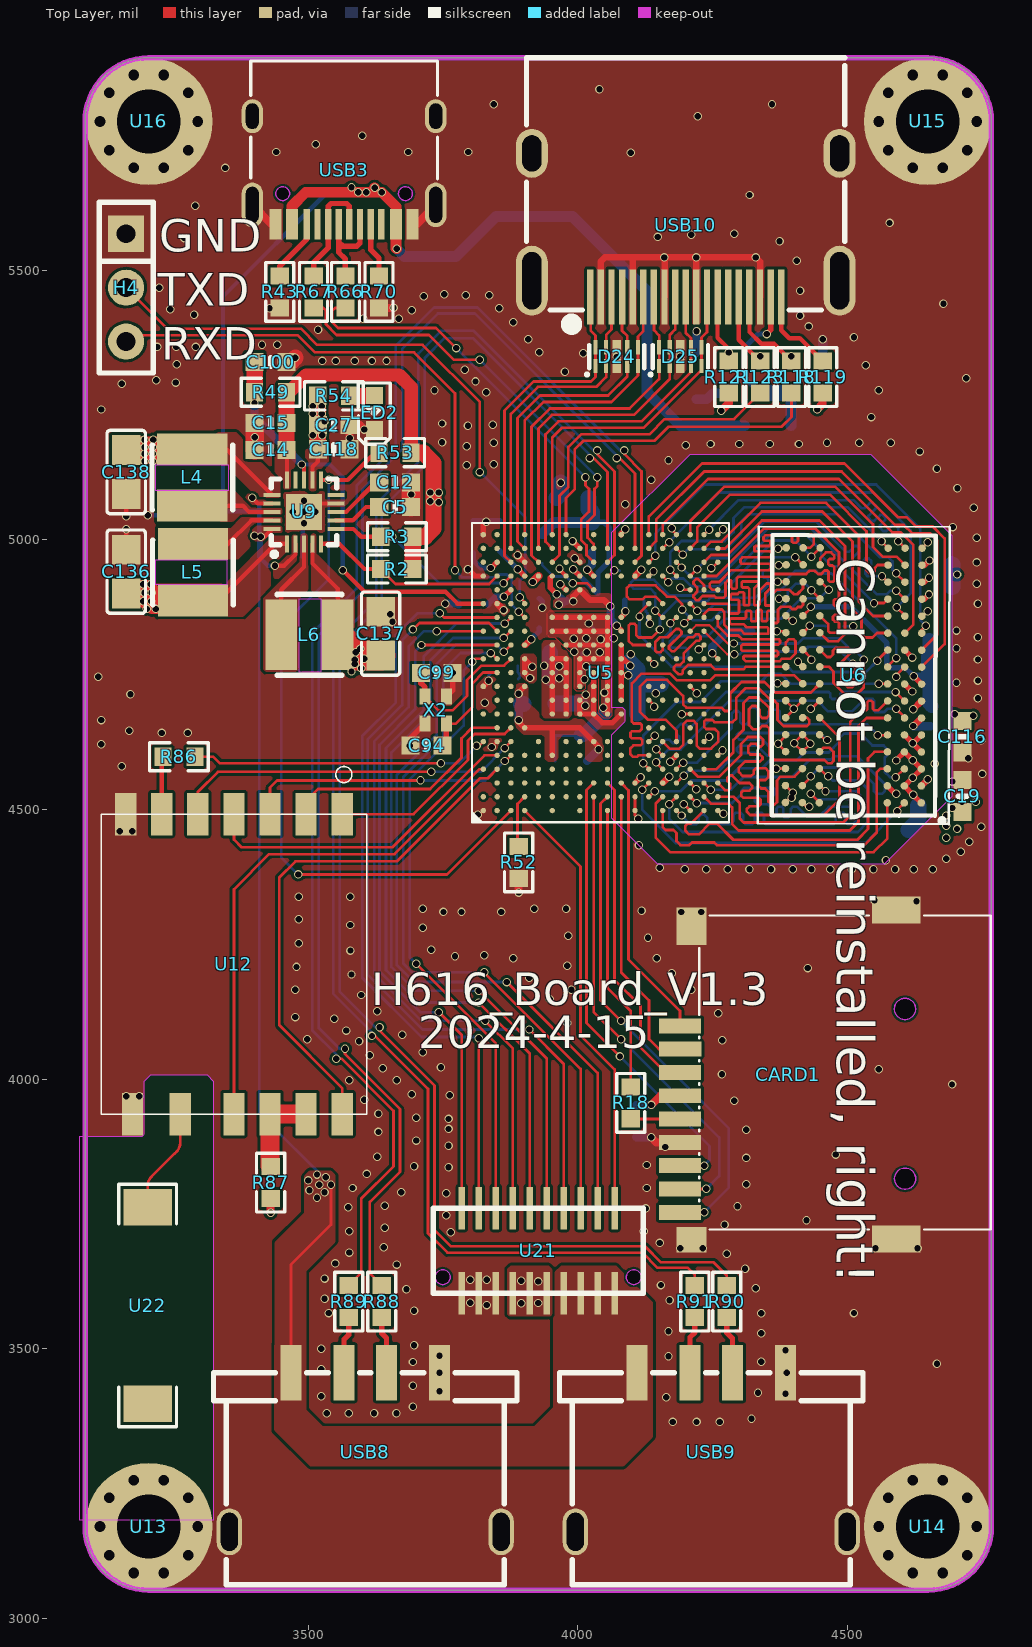
[diagram p0: Top Layer view]
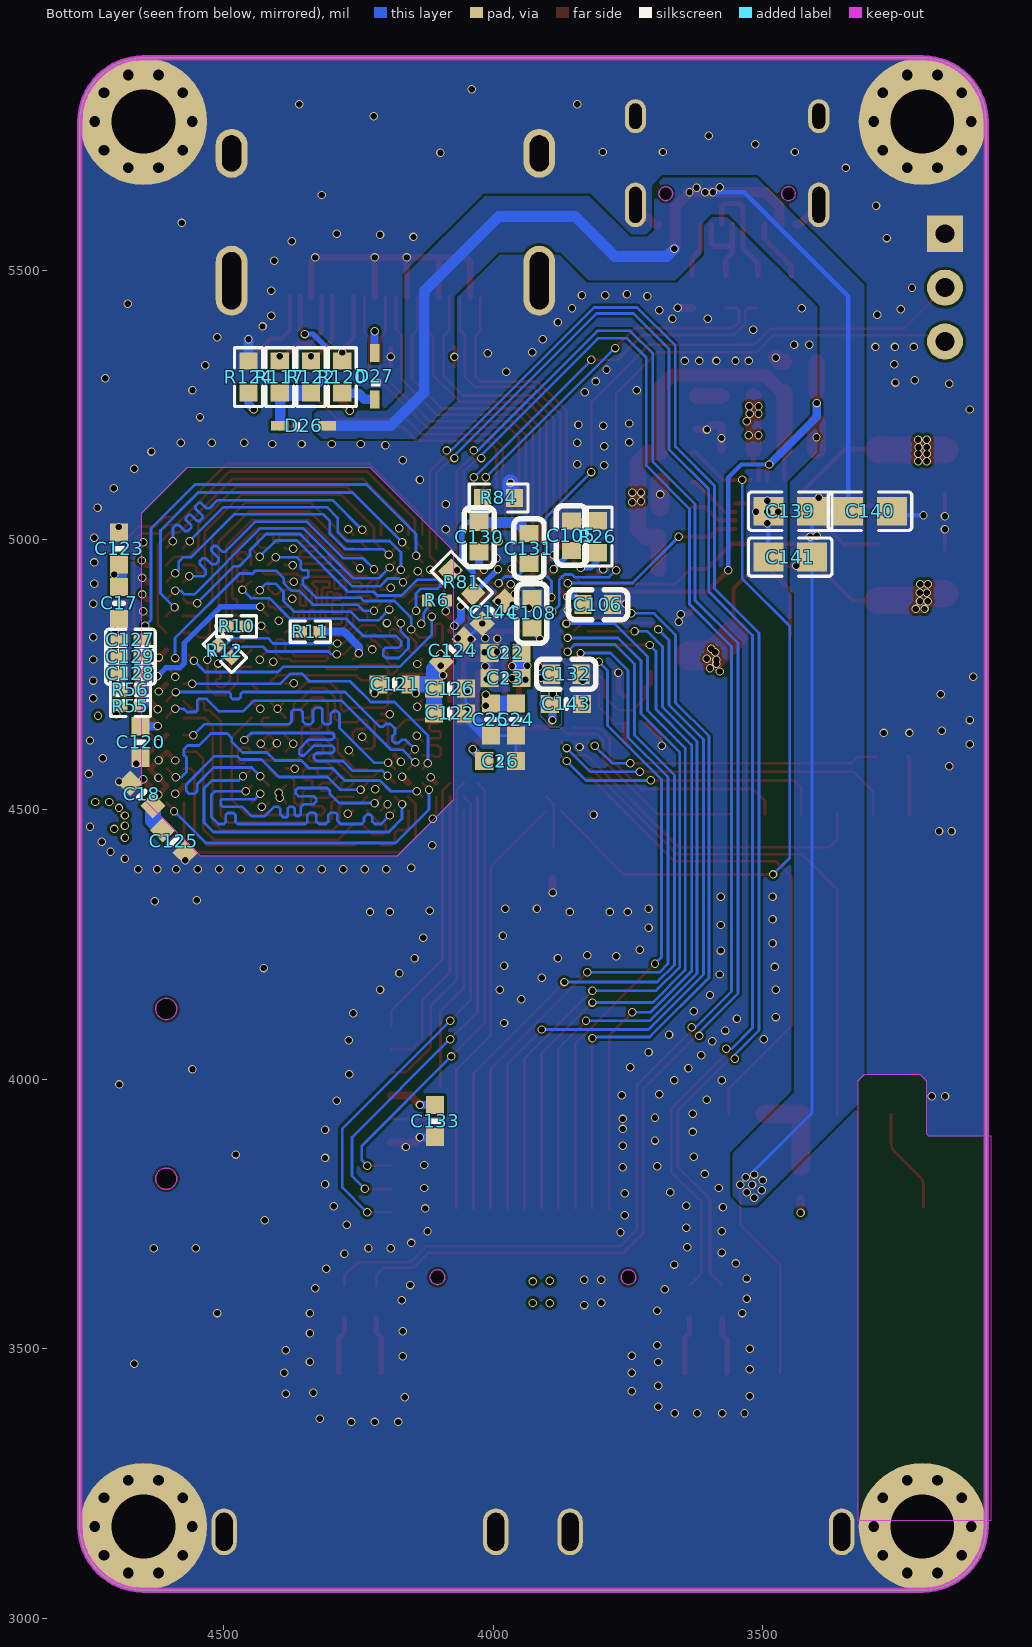
[diagram p1: Bottom Layer view, seen from below]
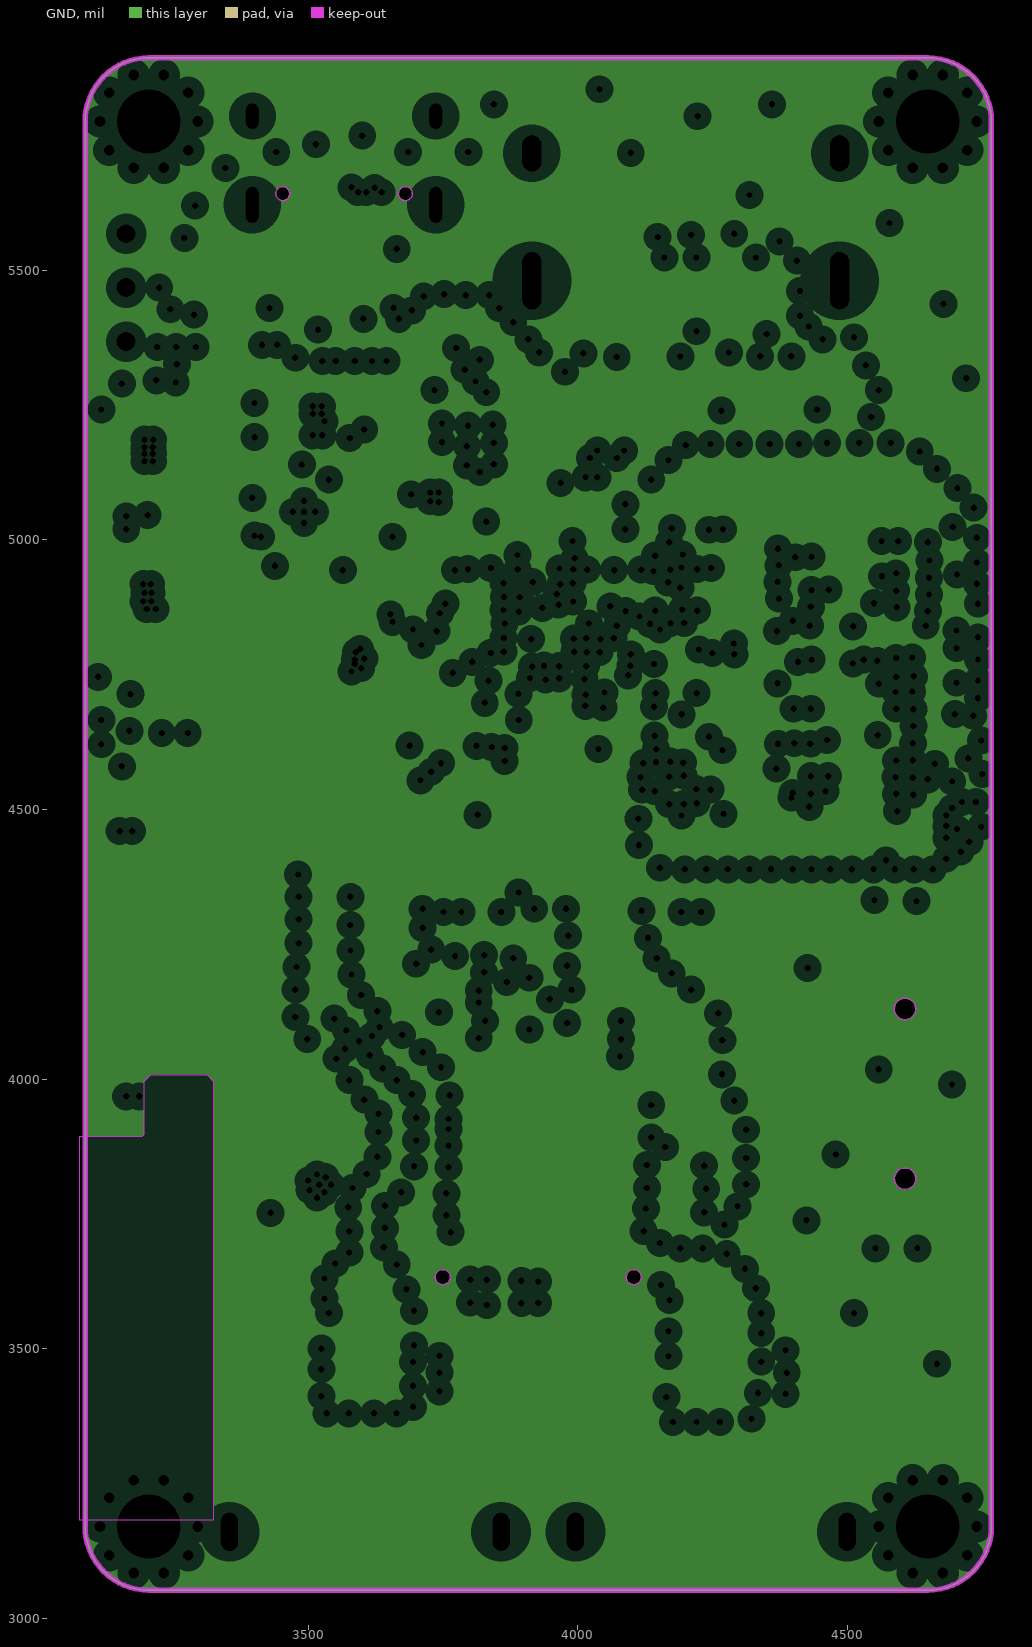
[diagram p2: GND, clearances drawn from the general rule]
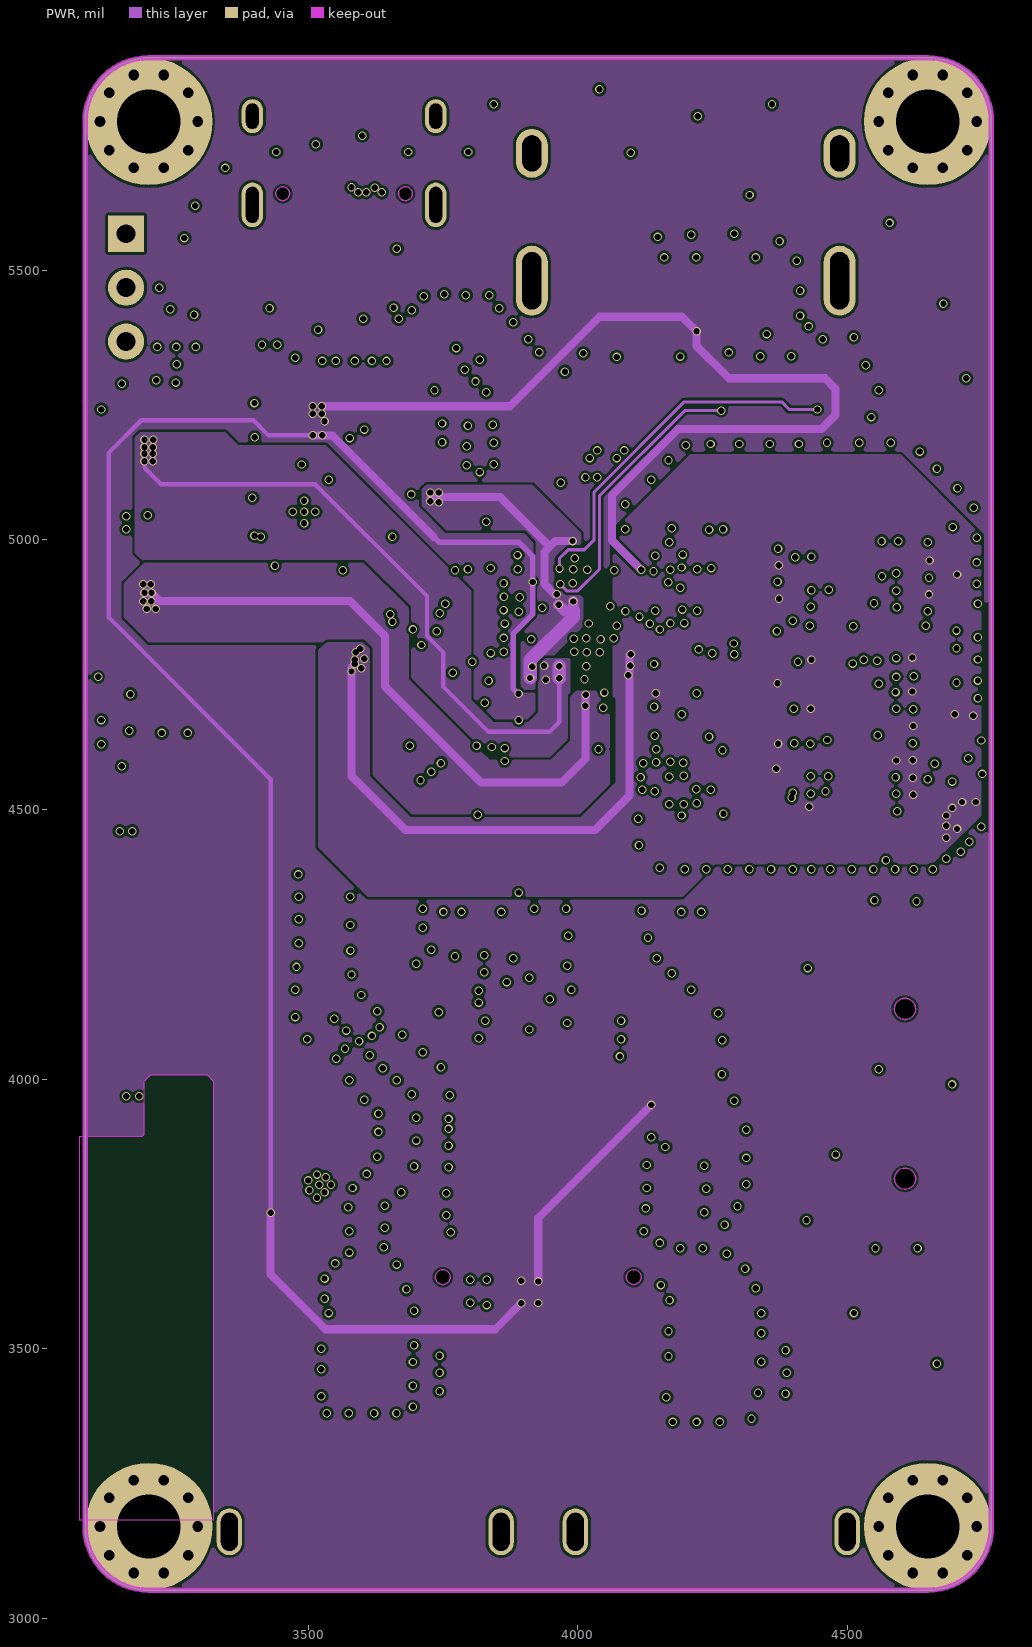
[diagram p3: PWR]
# Altium PCB MISC105417.pcbdoc (part 1 of 5)
Units mil, origin at the board's own origin, x right, y up, seen from the top; angles counter-clockwise.
Board outline 1681.1 x 2842.52 mil, 4 copper layers (Top Layer, GND, PWR, Bottom Layer), stack 62.447 mil thick; 102 components, 152 nets, 737 pads, 611 vias.

## Layer stack, top to bottom
Top Layer: signal copper 1.378
Dielectric1: surface 8.283, 7628 RC49% 8.6mil, Dk 0
GND: plane copper 0.598
Dielectric2: surface 41.929, 1.1mm H/HOZ 含铜, Dk 0
PWR: signal copper 0.598
Dielectric3: surface 8.283, 7628 RC49% 8.6mil, Dk 0
Bottom Layer: signal copper 1.378

## Board outline
3204,5894.41 ccw(c3204,5776.3) 3085.89,5776.3 3085.89,3170 ccw(c3204,3170) 3204,3051.89 4648.88,3051.89 ccw(c4648.88,3170) 4766.99,3170 4766.99,5776.3 ccw(c4648.88,5776.3) 4648.88,5894.41 3204,5894.41

## Design rules (kind name [scope] priority, off if disabled: settings)
BoardOutlineClearance safeClearance_1 [All] p2 off: genericclearance=3.5 ignorepadtopadclearanceinfootprint=FALSE except(0: Arc-SplitContinuation Track-SplitContinuation SMDPad-SplitContinuation THPad-SplitContinuation Via-SplitContinuation Fill-SplitContinuation Region-SplitContinuation Poly-SplitContinuation Text-SplitContinuation Hole-SplitContinuation; 4: Arc-OutlineEdge Track-OutlineEdge SMDPad-OutlineEdge THPad-OutlineEdge Via-OutlineEdge Fill-OutlineEdge Region-OutlineEdge Text-OutlineEdge Hole-OutlineEdge Arc-CutoutEdge Track-CutoutEdge SMDPad-CutoutEdge THPad-CutoutEdge Via-CutoutEdge Fill-CutoutEdge Region-CutoutEdge Text-CutoutEdge Hole-CutoutEdge; 5: Poly-OutlineEdge Poly-CutoutEdge)
BoardOutlineClearance copperThicknessInner0.5oz_1 [All] p4 off: genericclearance=3.5 ignorepadtopadclearanceinfootprint=FALSE except(0: Arc-SplitContinuation Track-SplitContinuation SMDPad-SplitContinuation THPad-SplitContinuation Via-SplitContinuation Fill-SplitContinuation Region-SplitContinuation Poly-SplitContinuation Text-SplitContinuation Hole-SplitContinuation; 4: Arc-OutlineEdge Track-OutlineEdge SMDPad-OutlineEdge THPad-OutlineEdge Via-OutlineEdge Fill-OutlineEdge Region-OutlineEdge Text-OutlineEdge Hole-OutlineEdge Arc-CutoutEdge Track-CutoutEdge SMDPad-CutoutEdge THPad-CutoutEdge Via-CutoutEdge Fill-CutoutEdge Region-CutoutEdge Text-CutoutEdge Hole-CutoutEdge; 5: Poly-OutlineEdge Poly-CutoutEdge)
BoardOutlineClearance Plane_innerPlane_1 [All] p6 off: genericclearance=4 ignorepadtopadclearanceinfootprint=FALSE except(0: Arc-SplitContinuation Track-SplitContinuation SMDPad-SplitContinuation THPad-SplitContinuation Via-SplitContinuation Fill-SplitContinuation Region-SplitContinuation Poly-SplitContinuation Text-SplitContinuation Hole-SplitContinuation; 4: Arc-OutlineEdge Track-OutlineEdge SMDPad-OutlineEdge THPad-OutlineEdge Via-OutlineEdge Fill-OutlineEdge Region-OutlineEdge Text-OutlineEdge Hole-OutlineEdge Arc-CutoutEdge Track-CutoutEdge SMDPad-CutoutEdge THPad-CutoutEdge Via-CutoutEdge Fill-CutoutEdge Region-CutoutEdge Text-CutoutEdge Hole-CutoutEdge; 5: Poly-OutlineEdge Poly-CutoutEdge)
BoardOutlineClearance Copper_copperRegion_1 [All] p8 off: genericclearance=4 ignorepadtopadclearanceinfootprint=FALSE except(0: Arc-SplitContinuation Track-SplitContinuation SMDPad-SplitContinuation THPad-SplitContinuation Via-SplitContinuation Fill-SplitContinuation Region-SplitContinuation Poly-SplitContinuation Text-SplitContinuation Hole-SplitContinuation; 4: Arc-OutlineEdge Track-OutlineEdge SMDPad-OutlineEdge THPad-OutlineEdge Via-OutlineEdge Fill-OutlineEdge Region-OutlineEdge Text-OutlineEdge Hole-OutlineEdge Arc-CutoutEdge Track-CutoutEdge SMDPad-CutoutEdge THPad-CutoutEdge Via-CutoutEdge Fill-CutoutEdge Region-CutoutEdge Text-CutoutEdge Hole-CutoutEdge; 10: Poly-OutlineEdge Poly-CutoutEdge)
BoardOutlineClearance Copper_近距离铺铜_1 [All] p10 off: genericclearance=4 ignorepadtopadclearanceinfootprint=FALSE except(0: Arc-SplitContinuation Track-SplitContinuation SMDPad-SplitContinuation THPad-SplitContinuation Via-SplitContinuation Fill-SplitContinuation Region-SplitContinuation Poly-SplitContinuation Text-SplitContinuation Hole-SplitContinuation; 4: Arc-OutlineEdge Track-OutlineEdge SMDPad-OutlineEdge THPad-OutlineEdge Via-OutlineEdge Fill-OutlineEdge Region-OutlineEdge Text-OutlineEdge Hole-OutlineEdge Arc-CutoutEdge Track-CutoutEdge SMDPad-CutoutEdge THPad-CutoutEdge Via-CutoutEdge Fill-CutoutEdge Region-CutoutEdge Text-CutoutEdge Hole-CutoutEdge; 5: Poly-OutlineEdge Poly-CutoutEdge)
BoardOutlineClearance Copper_发散铺铜_1 [All] p12 off: genericclearance=4 ignorepadtopadclearanceinfootprint=FALSE except(0: Arc-SplitContinuation Track-SplitContinuation SMDPad-SplitContinuation THPad-SplitContinuation Via-SplitContinuation Fill-SplitContinuation Region-SplitContinuation Poly-SplitContinuation Text-SplitContinuation Hole-SplitContinuation; 4: Arc-OutlineEdge Track-OutlineEdge SMDPad-OutlineEdge THPad-OutlineEdge Via-OutlineEdge Fill-OutlineEdge Region-OutlineEdge Text-OutlineEdge Hole-OutlineEdge Arc-CutoutEdge Track-CutoutEdge SMDPad-CutoutEdge THPad-CutoutEdge Via-CutoutEdge Fill-CutoutEdge Region-CutoutEdge Text-CutoutEdge Hole-CutoutEdge; 5: Poly-OutlineEdge Poly-CutoutEdge)
BoardOutlineClearance copperThickness1oz_1 [All] p14: genericclearance=4 ignorepadtopadclearanceinfootprint=FALSE except(0: Arc-SplitContinuation Track-SplitContinuation SMDPad-SplitContinuation THPad-SplitContinuation Via-SplitContinuation Fill-SplitContinuation Region-SplitContinuation Poly-SplitContinuation Text-SplitContinuation Hole-SplitContinuation; 4: Arc-OutlineEdge Track-OutlineEdge SMDPad-OutlineEdge THPad-OutlineEdge Via-OutlineEdge Fill-OutlineEdge Region-OutlineEdge Text-OutlineEdge Hole-OutlineEdge Arc-CutoutEdge Track-CutoutEdge SMDPad-CutoutEdge THPad-CutoutEdge Via-CutoutEdge Fill-CutoutEdge Region-CutoutEdge Text-CutoutEdge Hole-CutoutEdge; 5: Poly-OutlineEdge Poly-CutoutEdge)
Clearance safeClearance [All] p1 off: gap=3.5 ignorepadtopadclearanceinfootprint=FALSE except(4: Track-Via SMDPad-Via THPad-Via Via-Via Fill-Track Region-Track Fill-SMDPad Region-SMDPad Fill-THPad Region-THPad Fill-Via Region-Via Fill-Fill Fill-Region Region-Region Arc-Track Arc-SMDPad Arc-THPad Arc-Via Fill-Arc Region-Arc Arc-Arc Text-Track SMDPad-Text Text-THPad Text-Via Fill-Text Region-Text Arc-Text Text-Text Hole-Via Fill-Hole Region-Hole Hole-Arc Hole-Text; 5: Poly-Track Poly-SMDPad Poly-THPad Poly-Via Poly-Fill Poly-Region Poly-Poly Poly-Arc Poly-Text Poly-Hole)
Clearance copperThicknessInner0.5oz [All] p3 off: gap=3.5 ignorepadtopadclearanceinfootprint=FALSE except(4: SMDPad-Track SMDPad-SMDPad THPad-Track SMDPad-THPad THPad-THPad Track-Via SMDPad-Via THPad-Via Via-Via Fill-Track Region-Track Fill-SMDPad Region-SMDPad Fill-THPad Region-THPad Fill-Via Region-Via Fill-Fill Fill-Region Region-Region Arc-Track Arc-SMDPad Arc-THPad Arc-Via Fill-Arc Region-Arc Arc-Arc Text-Track SMDPad-Text Text-THPad Text-Via Fill-Text Region-Text Arc-Text Text-Text Hole-Track Hole-SMDPad Hole-THPad Hole-Via Fill-Hole Region-Hole Hole-Arc Hole-Text; 5: Poly-Track Poly-SMDPad Poly-THPad Poly-Via Poly-Fill Poly-Region Poly-Poly Poly-Arc Poly-Text Poly-Hole)
Clearance Plane_innerPlane [All] p5 off: gap=4 ignorepadtopadclearanceinfootprint=FALSE except(5: Poly-Track Poly-SMDPad Poly-THPad Poly-Via Poly-Fill Poly-Region Poly-Poly Poly-Arc Poly-Text Poly-Hole)
Clearance Copper_copperRegion [All] p7 off: gap=4 ignorepadtopadclearanceinfootprint=FALSE except(10: Poly-Track Poly-SMDPad Poly-THPad Poly-Via Poly-Fill Poly-Region Poly-Poly Poly-Arc Poly-Text Poly-Hole)
Clearance Copper_近距离铺铜 [All] p9 off: gap=4 ignorepadtopadclearanceinfootprint=FALSE except(5: Poly-Track Poly-SMDPad Poly-THPad Poly-Via Poly-Fill Poly-Region Poly-Poly Poly-Arc Poly-Text Poly-Hole)
Clearance Copper_发散铺铜 [All] p11 off: gap=4 ignorepadtopadclearanceinfootprint=FALSE except(5: Poly-Track Poly-SMDPad Poly-THPad Poly-Via Poly-Fill Poly-Region Poly-Poly Poly-Arc Poly-Text Poly-Hole)
Clearance copperThickness1oz [All] p13: gap=4 ignorepadtopadclearanceinfootprint=FALSE except(5: Poly-Track Poly-SMDPad Poly-THPad Poly-Via Poly-Fill Poly-Region Poly-Poly Poly-Arc Poly-Text Poly-Hole)
DiffPairsRouting nei [All] p1 off: maxlimit=7 minlimit=7 mostfreqgap=7 toplayer_minwidth=4 toplayer_prefwidth=4 toplayer_maxwidth=10 toplayer_mingap=7 toplayer_prefgap=7 toplayer_maxgap=7 midlayer1_minwidth=4 midlayer1_prefwidth=4 midlayer1_maxwidth=10 midlayer1_mingap=7 midlayer1_prefgap=7 midlayer1_maxgap=7 bottomlayer_minwidth=4 bottomlayer_prefwidth=4 bottomlayer_maxwidth=10 bottomlayer_mingap=7 bottomlayer_prefgap=7 bottomlayer_maxgap=7 maxuncoupledlength=5
DiffPairsRouting wai [All] p2: maxlimit=5 minlimit=5 mostfreqgap=5 toplayer_minwidth=4 toplayer_prefwidth=4 toplayer_maxwidth=100 toplayer_mingap=5 toplayer_prefgap=5 toplayer_maxgap=5 midlayer1_minwidth=4 midlayer1_prefwidth=4 midlayer1_maxwidth=100 midlayer1_mingap=5 midlayer1_prefgap=5 midlayer1_maxgap=5 bottomlayer_minwidth=4 bottomlayer_prefwidth=4 bottomlayer_maxwidth=100 bottomlayer_mingap=5 bottomlayer_prefgap=5 bottomlayer_maxgap=5 maxuncoupledlength=10
HoleToHoleClearance otherClearance [All] p1: gap=11.8 allowstackedmicrovias=TRUE
Length netLength [All] p1: minlimit=0 maxlimit=0
PasteMaskExpansion pasteMaskExpansion [All] p1: expansion=0
PlaneConnect innerPlane [All] p1: planeconnectstyle=Direct reliefexpansion=20 reliefentries=4 reliefconductorwidth=10 reliefairgap=10
PolygonConnect copperRegion [All] p1 off: connectstyle=Relief reliefconductorwidth=10 reliefentries=4 polygonreliefangle="90 Angle" airgapwidth=10 via.connectstyle=Relief via.reliefconductorwidth=10 via.reliefentries=4 via.polygonreliefangle="90 Angle" via.airgapwidth=10
PolygonConnect 发散铺铜 [All] p2 off: connectstyle=Direct reliefconductorwidth=10 reliefentries=4 polygonreliefangle="90 Angle" airgapwidth=10 smdpad.connectstyle=Relief smdpad.reliefconductorwidth=10 smdpad.reliefentries=4 smdpad.polygonreliefangle="90 Angle" smdpad.airgapwidth=4 via.connectstyle=Relief via.reliefconductorwidth=10 via.reliefentries=4 via.polygonreliefangle="90 Angle" via.airgapwidth=10
PolygonConnect 近距离铺铜 [All] p3: connectstyle=Direct reliefconductorwidth=10 reliefentries=4 polygonreliefangle="90 Angle" airgapwidth=10 via.connectstyle=Relief via.reliefconductorwidth=10 via.reliefentries=4 via.polygonreliefangle="90 Angle" via.airgapwidth=10
RoutingVias viaSize [All] p1: holewidth=11.8 width=15.7 viastyle="Through Hole" minholewidth=11.8 minwidth=15.7 maxholewidth=236.2 maxwidth=393.7
SolderMaskExpansion solderMaskExpansion [IsVia] p1: expansion=-1000 istentingtop=TRUE
SolderMaskExpansion solderMaskExpansion [All] p2: expansion=4 istentingtop=FALSE
Width trackWidth [All] p1 off: maxlimit=100 minlimit=4 preferedwidth=5
Width copperThickness2oz [All] p2 off: maxlimit=100 minlimit=4 preferedwidth=10
Width copperThickness0.5oz [All] p3 off: maxlimit=100 minlimit=4 preferedwidth=10
Width copperThickness1oz_2 [All] p4: maxlimit=100 minlimit=4 preferedwidth=5

## Components (designator, comment, footprint, x,y, rotation, side; value= is the part's Value field where it differs from the comment)
C5 "" "C0603 NSK" 3661,5061 r180 top
C12 "" "C0603 NSK" 3661,5107 r180 top
C14 "" "C0603 NSK" 3430,5167 r0 top
C15 "" "C0603 NSK" 3430,5217 r0 top
C17 "" "C0603 NSK" 4694.2,4882.94 r90 bottom
C18 "" "C0603 NSK" 4652.2,4527.94 r225 bottom
C19 "" "C0603 NSK" 4713.2,4524.94 r270 top
C22 "" "C0603 NSK" 3977.48,4790.68 r180 bottom
C23 "" "C0603 NSK" 3977.48,4743.94 r180 bottom
C24 "" "C0603 NSK" 3958.2,4666.98 r90 bottom
C25 "" "C0603 NSK" 4004.25,4666.98 r90 bottom
C26 "" "C0603 NSK" 3987.2,4589.94 r0 bottom
C27 "" "C0603 NSK" 3547,5213 r180 top
C94 "" "C0603 NSK" 3719.25,4618.45 r180 top
C99 "" "C0603 NSK" 3738.25,4753.45 r0 top
C100 "" "C0603 NSK" 3430,5330 r180 top
C105 "2.2UF" C0603 3855.2,5007.94 r270 bottom
C106 "1UF" C0603 3806.2,4879.94 r0 bottom
C108 "220NF" C0603 3928.52,4863.91 r90 bottom
C116 "" "C0603 NSK" 4713.2,4634.94 r90 top
C118 "" "C0603 NSK" 3547.16,5168.29 r180 top
C120 "" "C0603 NSK" 4654.2,4624.94 r90 bottom
C121 "" "C0603 NSK" 4183.07,4732.31 r180 bottom
C122 "" "C0603 NSK" 4080.47,4678.21 r0 bottom
C123 "" "C0603 NSK" 4694.2,4983.94 r270 bottom
C124 "" "C0603 NSK" 4075.2,4794.94 r315 bottom
C125 "" "C0603 NSK" 4592.29,4441 r45 bottom
C126 "" "C0603 NSK" 4080.47,4724.21 r0 bottom
C127 "100nF" C0402 4672.97,4814.66 r180 bottom
C128 "100nF" C0402 4672.97,4751.94 r180 bottom
C129 "100nF" C0402 4672.97,4782.94 r180 bottom
C130 "2.2uF" C0603 4026.2,5004.94 r270 bottom
C131 "2.2uF" C0603 3934,4984 r270 bottom
C132 "100nF" C0603 3864.52,4750.91 r180 bottom
C133 "" "C0603 NSK" 4108,3922 r90 bottom
C136 "47uF" C0805 3162.16,4941.29 r90 top
C137 "47uF" C0805 3634.16,4826.29 r270 top
C138 "47uF" C0805 3162.16,5126 r270 top
C139 "47uF" C0805 3449.19,5053.29 r180 bottom
C140 "47uF" C0805 3301.16,5053.29 r0 bottom
C141 "47uF" C0805 3449.19,4968.29 r180 bottom
C143 "" "C0603 NSK" 3864.82,4695.91 r0 bottom
C144 "" "C0603 NSK" 3999.52,4865.91 r135 bottom
CARD1 "TF-015" TF-SMD_TF-015 4390,4008 r90 top
D24 "" SLP2510P8_L2.5-W1.0-P0.50-BL 4072,5340 r0 top
D25 "" SLP2510P8_L2.5-W1.0-P0.50-BL 4190,5340 r0 top
D26 "" SOD-323_L1.8-W1.3-LS2.5-NSK 4352,5212 r180 bottom
D27 "" SOD-323_L1.8-W1.3-LS2.5-NSK 4220,5304 r90 bottom
H4 "" hdr-th_3p-p2.54-v-m 3162,5468 r270 top
L4 "1uH" IND-SMD_L3.0-W3.0 3285,5116 r270 top
L5 "1uH" IND-SMD_L3.0-W3.0 3286,4940 r90 top
L6 "1uH" IND-SMD_L3.0-W3.0 3502,4824 r180 top
LED2 "" LED_0603 3622.16,5238.29 r90 top
R2 "" R0603 3664,4946 r180 top
R3 "" R0603 3664,5006 r180 top
R6 "" R0402-NSK_2 4104.52,4887.91 r0 bottom
R10 "240" R0402 4476.2,4839.94 r180 bottom
R11 "240" R0402 4339.2,4829.94 r0 bottom
R12 "100" R0402 4497.73,4794.1 r45 bottom
R18 "10Ω" R0603 4098,3956 r270 top
R26 "6.04k" R0603 3806,5006 r90 bottom
R43 "" R0603 3447.03,5460.08 r270 top
R49 "" R0603 3430,5274 r0 top
R52 "" R0603 3890,4402 r270 top
R53 "" R0603 3661,5162 r180 top
R54 "10K" R0603 3547.16,5267.29 r180 top
R55 "2K" R0402 4672.97,4691.94 r180 bottom
R56 "2K" R0402 4672.97,4721.94 r0 bottom
R66 "22R" R0603 3568.75,5460.08 r90 top
R67 "10K" R0603 3509.7,5460.08 r90 top
R70 "" R0603 3631.03,5460.08 r90 top
R81 "150K" R0603 4058.2,4921.94 r45 bottom
R84 "0" R0603 3990.2,5077.94 r0 bottom
R86 "10Ω" R0603 3260,4598 r0 top
R87 "0Ω" R0603 3430,3808 r90 top
R88 "10K" R0603 3636.03,3587.32 r270 top
R89 "22R" R0603 3575.03,3587.32 r270 top
R90 "10K" R0603 4276.02,3587.32 r270 top
R91 "22R" R0603 4216.97,3587.32 r270 top
R117 "10k" R0603 4396,5302 r90 bottom
R118 "100" R0603 4396,5302 r90 top
R119 "510" R0603 4454,5302 r90 top
R120 "27k" R0603 4280,5302 r90 bottom
R121 "100" R0603 4280,5302 r90 top
R122 "10k" R0603 4338,5302 r90 bottom
R123 "100" R0603 4338,5302 r90 top
R124 "100k" R0603 4454,5302 r90 bottom
U5 "" BGA284P65B1200_1400H125 4042,4754 r90 top locked
U6 "" FBGA96 4509.2,4754 r179.8 top
U9 "AXP313A" WQFN-20_L3.0-W3.0-P0.40-BL-EP 3492,5052 r0 top
U12 "" WIFI模块 3608,4568 r270 top locked
U13 "" M3_HOLE 3204,3170 r0 top
U14 "" M3_HOLE 4648.88,3170 r0 top
U15 "" M3_HOLE 4648.88,5776.3 r0 top
U16 "" M3_HOLE 3204,5776.3 r0 top
U21 "" BTB2X10 3926.44,3681.81 r90 top locked
U22 "AN9520" ANT-SMD_L9.5-W2.1 3202,3580 r270 top locked
USB3 "" USB-C-SMD_TYPEC-304-BCP16-1 3566.2,5685.75 r180 top locked
USB8 "A/F board mount, type C, 10 (first two pins without curled edge), metal shell, LCP black glue=6.8" USB-A-SMD_C42496 3605.57,3307.8 r0 top locked
USB9 "A/F board mount, type C, 10 (first two pins without curled edge), metal shell, LCP black glue=6.8" USB-A-SMD_C42496 4247.31,3307.8 r0 top locked
USB10 "HDMI 19PIN 043" HDMI-SMD_HDMI-19PIN-043 4200,5584 r180 top locked
X2 "24M" OSC-SMD_4P-L2.0-W1.6-BL 3736.12,4684.35 r90 top

## Footprints (in the part's own frame and the unit in brackets; to place one, negate y for a bottom-side part, rotate by r counter-clockwise, add the part's x,y. Pads: shape width x height; smd on the part's side, far side on the other; paste and mask are expansions set on the pad)
ANT-SMD_L9.5-W2.1 [mm]
  rect 1.71x2.268 smd paste-100 mask+0.051: 1(-4.63,0) 2(4.63,0)
  silkscreen extent -5.71,-1.36 5.71,1.36
BGA284P65B1200_1400H125 [mil]
  round 10 smd paste+0.98 mask+1.97: A1(-255.91,217.52) A2(-230.31,217.52) A4(-179.13,217.52) A6(-127.95,217.52) A8(-76.77,217.52) A10(-25.59,217.52) A12(25.59,217.52) A14(76.77,217.52) A16(127.95,217.52) A18(179.13,217.52) A19(204.72,217.52) A20(230.31,217.52) A21(255.91,217.52) B1(-255.91,191.93) B2(-230.31,191.93) B3(-204.72,191.93) B4(-179.13,191.93) B5(-153.54,191.93) B6(-127.95,191.93) B7(-102.36,191.93) B8(-76.77,191.93) B9(-51.18,191.93) B10(-25.59,191.93) B11(0,191.93) B12(25.59,191.93) B13(51.18,191.93) B14(76.77,191.93) B15(102.36,191.93) B16(127.95,191.93) B17(153.54,191.93) B18(179.13,191.93) B19(204.72,191.93) B20(230.31,191.93) B21(255.91,191.93) C1(-255.91,166.34) C2(-230.31,166.34) C3(-204.72,166.34) C4(-179.13,166.34) C5(-153.54,166.34) C6(-127.95,166.34) C7(-102.36,166.34) C8(-76.77,166.34) C9(-51.18,166.34) C10(-25.59,166.34) C11(0,166.34) C12(25.59,166.34) C13(51.18,166.34) C14(76.77,166.34) C15(102.36,166.34) C16(127.95,166.34) C17(153.54,166.34) C18(179.13,166.34) C19(204.72,166.34) C20(230.31,166.34) D1(-255.91,140.75) D2(-230.31,140.75) D3(-204.72,140.75) D4(-179.13,140.75) D5(-153.54,140.75) D7(-102.36,140.75) D10(-25.59,140.75) D11(0,140.75) D12(25.59,140.75) D13(51.18,140.75) D14(76.77,140.75) D15(102.36,140.75) D16(127.95,140.75) D18(179.13,140.75) D19(204.72,140.75) D20(230.31,140.75) D21(255.91,140.75) E2(-230.31,115.16) E3(-204.72,115.16) E4(-179.13,115.16) E5(-153.54,115.16) E6(-127.95,115.16) E18(179.13,115.16) E19(204.72,115.16) E20(230.31,115.16) F1(-255.91,89.57) F2(-230.31,89.57) F3(-204.72,89.57) F4(-179.13,89.57) F5(-153.54,89.57) F8(-76.77,89.57) F9(-51.18,89.57) F10(-25.59,89.57) F11(0,89.57) F12(25.59,89.57) F13(51.18,89.57) F14(76.77,89.57) F15(102.36,89.57) F18(179.13,89.57) F19(204.72,89.57) F20(230.31,89.57) F21(255.91,89.57) G2(-230.31,63.98) G3(-204.72,63.98) G4(-179.13,63.98) G5(-153.54,63.98) G6(-127.95,63.98) G8(-76.77,63.98) G9(-51.18,63.98) G10(-25.59,63.98) G11(0,63.98) G12(25.59,63.98) G13(51.18,63.98) G14(76.77,63.98) G15(102.36,63.98) G17(153.54,63.98) G18(179.13,63.98) G19(204.72,63.98) G20(230.31,63.98) G21(255.91,63.98) H1(-255.91,38.39) H2(-230.31,38.39) H3(-204.72,38.39) H4(-179.13,38.39) H5(-153.54,38.39) H6(-127.95,38.39) H8(-76.77,38.39) H9(-51.18,38.39) H10(-25.59,38.39) H11(0,38.39) H12(25.59,38.39) H13(51.18,38.39) H14(76.77,38.39) H15(102.36,38.39) H17(153.54,38.39) H18(179.13,38.39) H19(204.72,38.39) H20(230.31,38.39) J2(-230.31,12.8) J3(-204.72,12.8) J6(-127.95,12.8) J8(-76.77,12.8) J9(-51.18,12.8) J10(-25.59,12.8) J11(0,12.8) J12(25.59,12.8) J13(51.18,12.8) J14(76.77,12.8) J15(102.36,12.8) J17(153.54,12.8) J18(179.13,12.8) J19(204.72,12.8) J20(230.31,12.8) J21(255.91,12.8) K1(-255.91,-12.8) K2(-230.31,-12.8) K3(-204.72,-12.8) K4(-179.13,-12.8) K5(-153.54,-12.8) K6(-127.95,-12.8) K8(-76.77,-12.8) K9(-51.18,-12.8) K10(-25.59,-12.8) K11(0,-12.8) K12(25.59,-12.8) K13(51.18,-12.8) K14(76.77,-12.8) K15(102.36,-12.8) K18(179.13,-12.8) K19(204.72,-12.8) K20(230.31,-12.8) L2(-230.31,-38.39) L3(-204.72,-38.39) L4(-179.13,-38.39) L5(-153.54,-38.39) L6(-127.95,-38.39) L8(-76.77,-38.39) L9(-51.18,-38.39) L10(-25.59,-38.39) L11(0,-38.39) L12(25.59,-38.39) L13(51.18,-38.39) L14(76.77,-38.39) L15(102.36,-38.39) L18(179.13,-38.39) L19(204.72,-38.39) L20(230.31,-38.39) L21(255.91,-38.39) M1(-255.91,-63.98) M2(-230.31,-63.98) M3(-204.72,-63.98) M18(179.13,-63.98) M19(204.72,-63.98) M20(230.31,-63.98) N2(-230.31,-89.57) N3(-204.72,-89.57) N4(-179.13,-89.57) N5(-153.54,-89.57) N6(-127.95,-89.57) N7(-102.36,-89.57) N9(-51.18,-89.57) N10(-25.59,-89.57) N12(25.59,-89.57) N13(51.18,-89.57) N15(102.36,-89.57) N16(127.95,-89.57) N18(179.13,-89.57) N19(204.72,-89.57) N20(230.31,-89.57) N21(255.91,-89.57) P1(-255.91,-115.16) P2(-230.31,-115.16) P3(-204.72,-115.16) P4(-179.13,-115.16) P5(-153.54,-115.16) P6(-127.95,-115.16) P7(-102.36,-115.16) P9(-51.18,-115.16) P10(-25.59,-115.16) P12(25.59,-115.16) P13(51.18,-115.16) P15(102.36,-115.16) P16(127.95,-115.16) P18(179.13,-115.16) P20(230.31,-115.16) P21(255.91,-115.16) R1(-255.91,-140.75) R2(-230.31,-140.75) R3(-204.72,-140.75) R4(-179.13,-140.75) R5(-153.54,-140.75) R6(-127.95,-140.75) R9(-51.18,-140.75) R12(25.59,-140.75) R15(102.36,-140.75) R18(179.13,-140.75) R19(204.72,-140.75) R20(230.31,-140.75) R21(255.91,-140.75) T1(-255.91,-166.34) T2(-230.31,-166.34) T3(-204.72,-166.34) T4(-179.13,-166.34) T5(-153.54,-166.34) T6(-127.95,-166.34) T7(-102.36,-166.34) T8(-76.77,-166.34) T9(-51.18,-166.34) T10(-25.59,-166.34) T11(0,-166.34) T12(25.59,-166.34) T14(76.77,-166.34) T15(102.36,-166.34) T16(127.95,-166.34) T17(153.54,-166.34) T18(179.13,-166.34) T20(230.31,-166.34) T21(255.91,-166.34) U1(-255.91,-191.93) U2(-230.31,-191.93) U3(-204.72,-191.93) U4(-179.13,-191.93) U5(-153.54,-191.93) U6(-127.95,-191.93) U8(-76.77,-191.93) U9(-51.18,-191.93) U10(-25.59,-191.93) U11(0,-191.93) U12(25.59,-191.93) U13(51.18,-191.93) U14(76.77,-191.93) U15(102.36,-191.93) U16(127.95,-191.93) U17(153.54,-191.93) U18(179.13,-191.93) U19(204.72,-191.93) U20(230.31,-191.93) U21(255.91,-191.93) V1(-255.91,-217.52) V2(-230.31,-217.52) V3(-204.72,-217.52) V5(-153.54,-217.52) V8(-76.77,-217.52) V10(-25.59,-217.52) V12(25.59,-217.52) V15(102.36,-217.52) V17(153.54,-217.52) V19(204.72,-217.52) V20(230.31,-217.52) V21(255.91,-217.52)
  silkscreen extent -278,-238 278,238
BTB2X10 [mm]
  rect 2x0.3 smd: 1(-2,3.6) 2(-2,2.8) 3(-2,2) 4(-2,1.2) 5(-2,0.4) 6(-2,-0.4) 7(-2,-1.2) 8(-2,-2) 9(-2,-2.8) 10(-2,-3.6) 11(2,-3.6) 12(2,-2.8) 13(2,-2) 14(2,-1.2) 15(2,-0.4) 16(2,0.4) 17(2,1.2) 18(2,2) 19(2,2.8) 20(2,3.6)
  Board Outline Layer circle w0.003: c-1.25,4.5 r0.35
  Board Outline Layer circle w0.003: c-1.25,-4.5 r0.35
  Board Outline Layer region: -1.25,4.15 -1.402,4.185 -1.524,4.282 -1.591,4.422 -1.591,4.578 -1.524,4.718 -1.402,4.815 -1.25,4.85 -1.25,4.85 -1.098,4.815 -0.976,4.718 -0.909,4.578 -0.909,4.422 -0.976,4.282 -1.098,4.185 -1.25,4.15
  Board Outline Layer region: -1.25,4.15 -1.328,4.159 -1.402,4.185 -1.468,4.226 -1.524,4.282 -1.565,4.348 -1.591,4.422 -1.6,4.5 -1.591,4.578 -1.565,4.652 -1.524,4.718 -1.468,4.774 -1.402,4.815 -1.328,4.841 -1.25,4.85 -1.172,4.841 -1.098,4.815 -1.032,4.774 -0.976,4.718 -0.935,4.652 -0.909,4.578 -0.9,4.5 -0.909,4.422 -0.935,4.348 -0.976,4.282 -1.032,4.226 -1.098,4.185 -1.172,4.159
  Board Outline Layer region: -1.25,-4.85 -1.402,-4.815 -1.524,-4.718 -1.591,-4.578 -1.591,-4.422 -1.524,-4.282 -1.402,-4.185 -1.25,-4.15 -1.25,-4.15 -1.098,-4.185 -0.976,-4.282 -0.909,-4.422 -0.909,-4.578 -0.976,-4.718 -1.098,-4.815 -1.25,-4.85
  Board Outline Layer region: -1.25,-4.85 -1.328,-4.841 -1.402,-4.815 -1.468,-4.774 -1.524,-4.718 -1.565,-4.652 -1.591,-4.578 -1.6,-4.5 -1.591,-4.422 -1.565,-4.348 -1.524,-4.282 -1.468,-4.226 -1.402,-4.185 -1.328,-4.159 -1.25,-4.15 -1.172,-4.159 -1.098,-4.185 -1.032,-4.226 -0.976,-4.282 -0.935,-4.348 -0.909,-4.422 -0.9,-4.5 -0.909,-4.578 -0.935,-4.652 -0.976,-4.718 -1.032,-4.774 -1.098,-4.815 -1.172,-4.841
  Multi-Layer board cut-out: -1.25,4.15 -1.402,4.185 -1.524,4.282 -1.591,4.422 -1.591,4.578 -1.524,4.718 -1.402,4.815 -1.25,4.85 -1.25,4.85 -1.098,4.815 -0.976,4.718 -0.909,4.578 -0.909,4.422 -0.976,4.282 -1.098,4.185 -1.25,4.15
  Multi-Layer board cut-out: -1.25,-4.85 -1.402,-4.815 -1.524,-4.718 -1.591,-4.578 -1.591,-4.422 -1.524,-4.282 -1.402,-4.185 -1.25,-4.15 -1.25,-4.15 -1.098,-4.185 -0.976,-4.282 -0.909,-4.422 -0.909,-4.578 -0.976,-4.718 -1.098,-4.815 -1.25,-4.85
  silkscreen extent -2,-4.95 2,4.95
C0402 [mm]
  rect 0.79x0.54 smd paste-100 mask+0.051: 1(-0.545,0) 2(0.545,0)
  silkscreen extent -1.17,-0.5 1.17,0.5
C0603 [mm]
  rect 0.8x0.9 smd paste+0 mask+0.051: 1(-0.7,0) 2(0.7,0)
  silkscreen extent -1.41,-0.71 1.39,0.72
"C0603 NSK" [mm]
  rect 0.85x0.85 smd paste+0 mask+0.051: 1(-0.75,0) 2(0.75,0)
  silkscreen extent 0,-0.21 0,0.21
C0805 [mm]
  rect 1.41x1.35 smd paste-100 mask+0.051: 1(-1.03,0) 2(1.03,0)
  silkscreen extent -1.96,-0.9 1.96,0.9